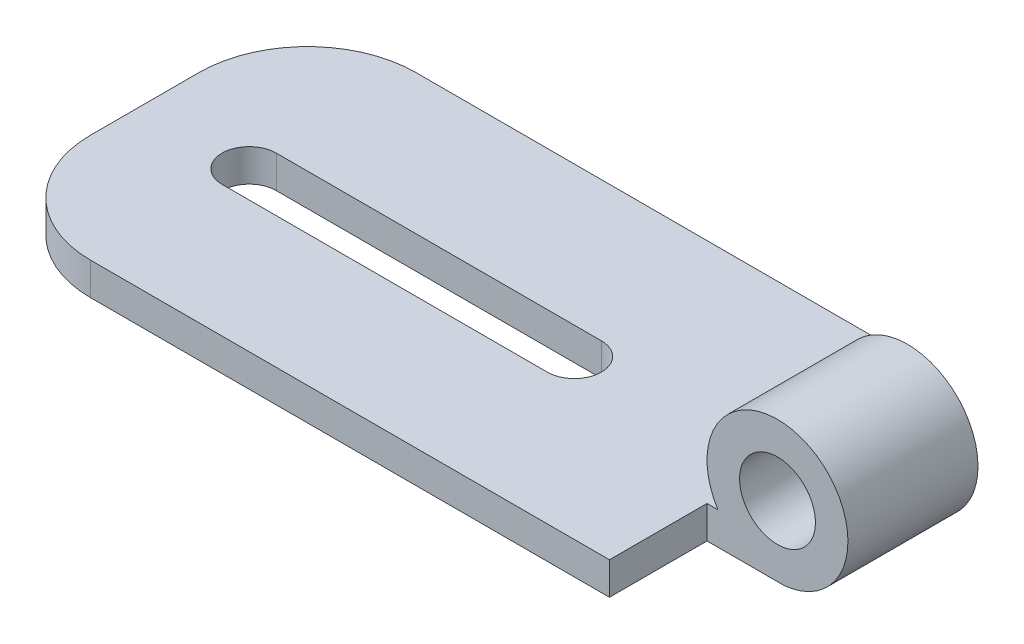
SolidWorks part; units mm, degrees
ref_plane "前视基准面" through (0, 0, 0) normal (0, 0, 1) x (1, 0, 0)
ref_plane "上视基准面" through (0, 0, 0) normal (0, 1, 0) x (1, 0, 0)
ref_plane "右视基准面" through (0, 0, 0) normal (1, 0, 0) x (0, 0, -1)
sketch "草图1" plane through (0, 0, 0) normal (0, 0, 1) x (1, 0, 0)
  line L1 (-32.5, 1.5) -> (26.3676, 1.5)
  line L2 (-32.5, 1.5) -> (-32.5, -1.5)
  line L3 (-32.5, -1.5) -> (32.5, -1.5)
  line L5 (-32.5, 1.5) -> (32.5, -1.5) construction
  line L6 (-32.5, -1.5) -> (26.5507, 1.2254) construction
  arc A0 (32.5, -1.5) -> (26.3676, 1.5) centre (31.8646, 4.9689) ccw
  circle A1 centre (31.8646, 4.9689) radius 3.5
  circle A2 centre (31.8646, 4.9689) radius 6.5 construction
  point P0 (0, 0)
  dimension "D2" = 13
  dimension "D4" = 3
extrude "凸台-拉伸1" add sketch "草图1" along normal blind 30
fillet "圆角1" radius 10 2 edges at (-32.5, 0, 0) (-32.5, 0, 30)
sketch "草图2" plane through (0, 1.5, 0) normal (0, 1, 0) x (1, 0, 0)
  line L0 (-32.5, -20) -> (-32.5, -10) construction
  line L1 (-22.5, -12.8776) -> (7.5, -12.8776)
  line L3 (-22.5, -17.8776) -> (7.5, -17.8776)
  line L5 (-22.5, -12.8776) -> (7.5, -17.8776) construction
  line L6 (-22.5, -17.8776) -> (7.5, -12.8776) construction
  arc A0 (7.5, -12.8776) -> (7.5, -17.8776) centre (7.5, -15.3776) cw
  arc A1 (-22.5, -17.8776) -> (-22.5, -12.8776) centre (-22.5, -15.3776) cw
  point P0 (-7.5, -15.3776)
  dimension "D1" = 5
  dimension "D2" = 30
  dimension "D3" = 25
extrude "切除-拉伸1" cut sketch "草图2" against normal blind 30
sketch "草图3" plane through (0, 1.5, 0) normal (0, 1, 0) x (1, 0, 0)
  line L2 (25.3646, -21) -> (25.3646, -30)
  line L3 (25.3646, -30) -> (43.9373, -30)
  line L4 (43.9373, -21) -> (43.9373, -30)
  line L5 (25.3646, -21) -> (43.9373, -30) construction
  line L6 (25.3646, -30) -> (43.9373, -21) construction
  line L7 (25.3646, 0) -> (25.3646, -30) construction
  line L8 (25.3646, -30) -> (38.3646, -30) construction
  line L9 (25.3646, 0) -> (53.8871, 0)
  line L10 (25.3646, 0) -> (25.3646, -9)
  line L11 (25.3646, -9) -> (53.8871, -9)
  line L12 (53.8871, 0) -> (53.8871, -9)
  line L13 (25.3646, -21) -> (43.9373, -21)
  point P0 (34.6509, -25.5)
  dimension "D1" = 9
  dimension "D2" = 9
  dimension "D3" = 9
extrude "切除-拉伸2" cut sketch "草图3" against normal mid plane 30
